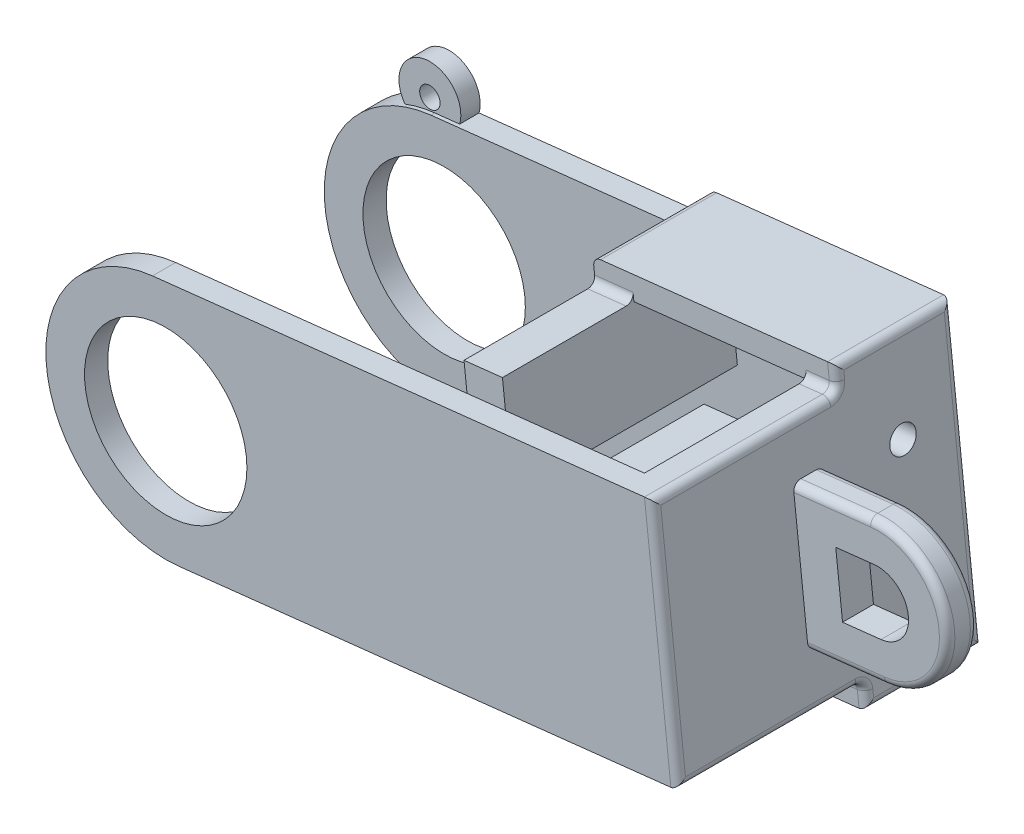
from build123d import *

# Parameters (mm, degrees)
SKETCH1_R                   = 21
BOSS_EXTRUDE1_DEPTH         = 6
BOSS_EXTRUDE2_DEPTH         = 78
SKETCH3_R                   = 3.0000000000000013
BOSS_EXTRUDE3_DEPTH         = 28
BOSS_EXTRUDE4_DEPTH         = 71.00000000000003
SKETCH10_R                  = 3.9999999999999982
BOSS_EXTRUDE6_DEPTH         = 1
CUT_EXTRUDE1_DEPTH          = 8
SKETCH8_W                   = 66
SKETCH8_H                   = 6.000000000000007
CUT_EXTRUDE3_DEPTH          = 15
BOSS_EXTRUDE7_DEPTH         = 6
FILLET2_R                   = 2
TAP_DRILL_FOR_M8_TAP1_D     = 6.8
TAP_DRILL_FOR_M8_TAP1_DEPTH = 20
TAP_DRILL_FOR_M8_TAP1_TIP   = 2.042926104693705
SKETCH14_R                  = 8
SKETCH14_R_2                = 2.6393435591760683
SKETCH14_R_3                = 2.7500000000000004
BOSS_EXTRUDE8_DEPTH         = 5
BOSS_EXTRUDE9_DEPTH         = 20
SKETCH16_R                  = 17.999999999999996
BOSS_EXTRUDE10_DEPTH        = 8
CUT_EXTRUDE4_DEPTH          = 8
FILLET3_R                   = 2


with BuildPart() as part:
    # Sketch1 → Boss-Extrude1 (new body)
    with BuildSketch(Plane.XY):
        with BuildLine():
            Line((132.62380505793305, -16.490188960571935), (3.41503919990868, -30.811321089221206))
            ThreePointArc((3.41503919990868, -30.811321089221206), (-30.81132108922119, -3.4150391999086844), (-3.415039199908666, 30.811321089221195))
            Line((-3.415039199908666, 30.811321089221195), (125.79372665811573, 45.132453217870456))
            Line((125.79372665811573, 45.132453217870456), (132.62380505793305, -16.490188960571935))
        make_face()
        Circle(SKETCH1_R, mode=Mode.SUBTRACT)
    extrude(amount=-BOSS_EXTRUDE1_DEPTH)

    # Sketch2 → Boss-Extrude2 (add)
    with BuildSketch(Plane.XY):
        Polygon((125.79372665811573, 45.132453217870456), (132.62380505793305, -16.49018896057193), (124.62761225366665, -17.376464229247457), (117.79753385384927, 44.24617794919492), align=None)
    extrude(amount=-BOSS_EXTRUDE2_DEPTH)

    # Sketch3 → Boss-Extrude3 (add)
    with BuildSketch(Plane(origin=(0, 0, -6), x_dir=(-1, 0, 0), z_dir=(0, 0, -1))):
        with Locations(Location((-50.00000000000005, 5.889675971997146, 0), (0, 0, 180))):
            Circle(SKETCH3_R)
    extrude(amount=BOSS_EXTRUDE3_DEPTH)

    # Sketch4 → Boss-Extrude4 (add)
    with BuildSketch(Plane(origin=(0, 0, -6), x_dir=(-1, 0, 0), z_dir=(0, 0, -1))):
        Polygon((-73.07142259530238, 39.28886298158555), (-79.90150099511973, -22.333779196856817), (-69.96236515988706, -23.435404745214456), (-63.132286760069725, 38.187237433227914), align=None)
    extrude(amount=BOSS_EXTRUDE4_DEPTH)

    # Sketch10 → Boss-Extrude6 (add)
    with BuildSketch(Plane(origin=(0, 0, -34), x_dir=(-1, 0, 0), z_dir=(0, 0, -1))):
        with Locations((-50.00000000000005, 5.889675971997146)):
            Circle(SKETCH10_R)
    extrude(amount=-BOSS_EXTRUDE6_DEPTH)

    # Mirror1: part across plane


with BuildPart() as part_1:
    add(part.part)
    add(part.part.mirror(Plane.XY.offset(-39)))

    # Sketch6 → Cut-Extrude1 (cut)
    with BuildSketch(Plane(origin=(0, 0, -6), x_dir=(-1, 0, 0), z_dir=(0, 0, -1))):
        Polygon((-77.79892131409314, 39.8128454942288), (-50.532545288662256, 36.79071792311109), (-51.836223102446034, 25.02861700243648), (-77.79892131409314, 27.90624863242818), align=None)
    cut_extrude1 = extrude(amount=CUT_EXTRUDE1_DEPTH, mode=Mode.SUBTRACT)

    # Mirror4: Cut-Extrude1 across plane
    add(cut_extrude1.mirror(Plane(origin=(0, 0, 0), x_dir=(0, 0, 1), z_dir=(-0.11016255483576362, 0.9939135835232646, 0))), mode=Mode.SUBTRACT)

    # Sketch8 → Cut-Extrude3 (cut)
    with BuildSketch(Plane(origin=(66.54732595997841, 7.375916344006741, 0), x_dir=(0, 0, 1), z_dir=(-0.9939135835232656, -0.1101625548357545, 0))):
        with Locations((-39, 2.9999999999999964)):
            Rectangle(SKETCH8_W, SKETCH8_H)
    cut_extrude3 = extrude(amount=-CUT_EXTRUDE3_DEPTH, mode=Mode.SUBTRACT)

    # Mirror5: Cut-Extrude3 across plane
    add(cut_extrude3.mirror(Plane(origin=(81.45602971282739, 9.02835466654305, -72), x_dir=(0, 0, 1), z_dir=(0.1101625548357545, -0.9939135835232656, 0))), mode=Mode.SUBTRACT)

    # Sketch11 → Boss-Extrude7 (add)
    with BuildSketch(Plane(origin=(-3.41503919990867, 30.811321089221206, 0), x_dir=(0.9939135835232645, 0.11016255483576355, 0), z_dir=(-0.11016255483576357, 0.9939135835232646, 0))):
        Polygon((129.99999999999997, 78), (66.95484100748354, 78), (66.95484100748354, 47.99999999999999), (129.99999999999997, 48), align=None)
    boss_extrude7 = extrude(amount=BOSS_EXTRUDE7_DEPTH)

    # Mirror6: Boss-Extrude7 across plane
    add(boss_extrude7.mirror(Plane(origin=(0, 0, 0), x_dir=(0, 0, 1), z_dir=(-0.11016255483576362, 0.9939135835232646, 0))))

    # Fillet2
    fillet2_edges = [part_1.edges().sort_by_distance(p)[0] for p in [
        (129.20876585802438, 14.321132128649257, -78),
        (125.79372665811574, 45.132453217870456, -24),
        (125.46323899360841, 48.114193968440254, -48),
        (68.10185467768603, 38.73805020740676, -47.99999999999999),
        (121.79563025598249, 44.689315583532704, -48),
        (125.13275132910113, 51.09593471901005, -63),
        (62.47131143105514, 44.15071893436753, -63),
        (132.62380505793305, -16.49018896057193, -24),
        (133.28478038694766, -22.45367046171154, -63),
        (132.95429272244036, -19.471929711141737, -48),
        (70.62334048890166, -29.39888624635408, -63),
        (74.9319330775034, -22.884591971035665, -47.99999999999999),
        (128.62570865579985, -16.933326594909712, -48),
        (129.20876585802438, 14.32113212864926, 0),
    ]]
    fillet(fillet2_edges, radius=FILLET2_R)

    # Tap Drill for M8 Tap1
    with Locations(Plane(origin=(129.2087658580244, 14.321132128649255, 0), x_dir=(0, 0, -1), z_dir=(0.9939135835232646, 0.11016255483576352, 0))):
        with Locations((63, 14), (63, -16)):
            Hole(TAP_DRILL_FOR_M8_TAP1_D / 2, depth=TAP_DRILL_FOR_M8_TAP1_DEPTH)
            with Locations((0, 0, -(TAP_DRILL_FOR_M8_TAP1_DEPTH + TAP_DRILL_FOR_M8_TAP1_TIP / 2))):  # 118° drill point
                Cone(0, TAP_DRILL_FOR_M8_TAP1_D / 2, TAP_DRILL_FOR_M8_TAP1_TIP, mode=Mode.SUBTRACT)

    # Sketch14 → Boss-Extrude8 (add)
    # profile 1 of 2: a face of its own
    with BuildSketch(Plane(origin=(0, 0, -78), x_dir=(-1, 0, 0), z_dir=(0, 0, -1))):
        with Locations((4.683649461628586, 33.67585823287338)):
            Circle(SKETCH14_R)
        with Locations((4.683649461628586, 33.67585823287338)):
            Circle(SKETCH14_R_2, mode=Mode.SUBTRACT)
    # profile 2 of 2: a face of its own
    with BuildSketch(Plane(origin=(0, 0, -78), x_dir=(-1, 0, 0), z_dir=(0, 0, -1))):
        with Locations((-4.683649461628697, -33.675858232873395)):
            Circle(SKETCH14_R)
        with Locations((-4.683649461628697, -33.675858232873395)):
            Circle(SKETCH14_R_3, mode=Mode.SUBTRACT)
    extrude(amount=-BOSS_EXTRUDE8_DEPTH)

    # Sketch15 → Boss-Extrude9 (add)
    with BuildSketch(Plane(origin=(129.2087658580244, 14.321132128649255, 0), x_dir=(0, 0, -1), z_dir=(0.9939135835232646, 0.11016255483576352, 0))):
        Polygon((43, -17.999999999999993), (34.999999999999865, -18), (34.999999999999865, 18), (43, 18.000000000000007), align=None)
    extrude(amount=BOSS_EXTRUDE9_DEPTH)

    # Sketch16 → Boss-Extrude10 (add)
    with BuildSketch(Plane(origin=(0, 0, -43), x_dir=(-1, 0, 0), z_dir=(0, 0, -1))):
        with Locations((-149.0870375284897, 16.524383225364534)):
            Circle(SKETCH16_R)
    extrude(amount=-BOSS_EXTRUDE10_DEPTH)

    # Sketch17 → Cut-Extrude4 (cut)
    with BuildSketch(Plane(origin=(0, 0, -43), x_dir=(-1, 0, 0), z_dir=(0, 0, -1))):
        with BuildLine():
            Line((-138.26660125457093, 23.374066345193015), (-148.20573708980362, 24.475691893550643))
            ThreePointArc((-148.20573708980362, 24.475691893550643), (-157.0383461966758, 17.40568366405063), (-149.9683379671758, 8.573074557178417))
            Line((-149.9683379671758, 8.573074557178417), (-140.02920213194318, 7.471449008820779))
            Line((-140.02920213194318, 7.471449008820779), (-138.26660125457093, 23.374066345193015))
        make_face()
    extrude(amount=-CUT_EXTRUDE4_DEPTH, mode=Mode.SUBTRACT)

    # Fillet3
    fillet3_edges = [part_1.edges().sort_by_distance(p)[0] for p in [
        (137.1649757062133, 33.31320218042565, -34.999999999999865),
        (141.1308276803008, -2.4676868264118728, -34.999999999999865),
        (141.13082768030077, -2.4676868264118657, -43),
        (137.1649757062133, 33.31320218042566, -43),
        (166.97748203190847, 18.507309212408288, -35),
        (166.97748203190847, 18.507309212408288, -43),
    ]]
    fillet(fillet3_edges, radius=FILLET3_R)


solid = part_1.part
